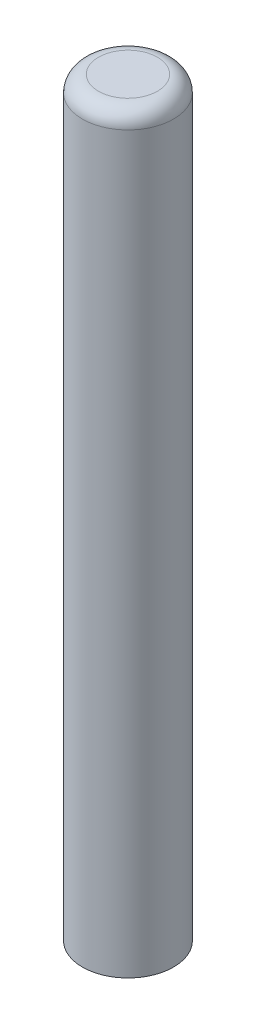
SolidWorks part; units mm, degrees
ref_plane "Front Plane" through (0, 0, 0) normal (0, 0, 1) x (1, 0, 0)
ref_plane "Top Plane" through (0, 0, 0) normal (0, 1, 0) x (1, 0, 0)
ref_plane "Right Plane" through (0, 0, 0) normal (1, 0, 0) x (0, 0, -1)
sketch "Sketch1" plane through (0, 0, 0) normal (0, 1, 0) x (1, 0, 0)
  circle A0 centre (0, 0) radius 4.25
extrude "Boss-Extrude1" add sketch "Sketch1" along normal blind 70
fillet "Fillet1" radius 1.5 1 edges at (0, 70, 4.25)
